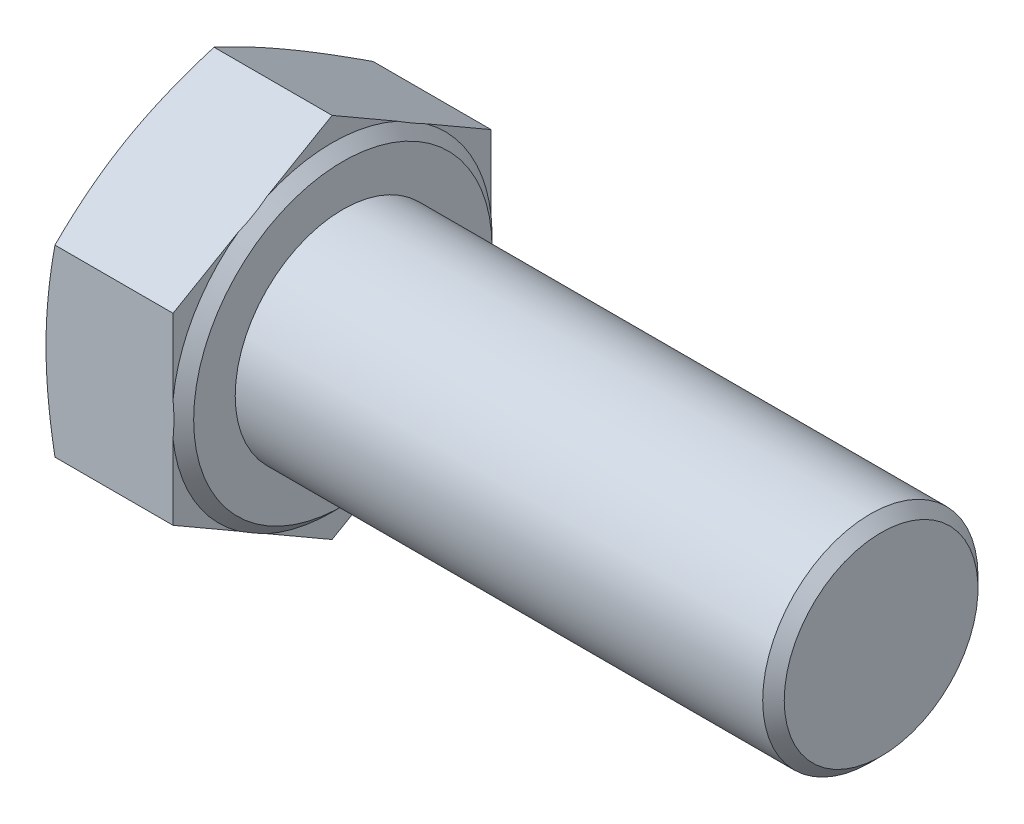
SolidWorks part; units mm, degrees
ref_plane "Front" through (0, 0, 0) normal (0, 0, 1) x (1, 0, 0)
ref_plane "Top" through (0, 0, 0) normal (0, 1, 0) x (1, 0, 0)
ref_plane "Right" through (0, 0, 0) normal (1, 0, 0) x (0, 0, -1)
other "Configuration Table"
sketch "Sketch2" plane through (0, 0, 0) normal (1, 0, 0) x (0, 0, -1)
  line L1 (8.865, -5.1182) -> (8.865, 5.1182)
  line L2 (8.865, 5.1182) -> (0, 10.2364)
  line L3 (0, 10.2364) -> (-8.865, 5.1182)
  line L4 (-8.865, 5.1182) -> (-8.865, -5.1182)
  line L5 (-8.865, -5.1182) -> (0, -10.2364)
  line L6 (0, -10.2364) -> (8.865, -5.1182)
  circle A0 centre (0, 0) radius 8.865 construction
extrude "BaseHead" add sketch "Sketch2" along normal blind 7.68
sketch "Sketch3" plane through (0, 0, 0) normal (0, 0, 1) x (1, 0, 0)
  line L0 (7.68, 10.2364) -> (7.68, 8.315)
  line L2 (7.68, 8.315) -> (7.08, 8.915)
  line L3 (7.08, 8.915) -> (7.08, 10.2364)
  line L5 (7.08, 10.2364) -> (7.68, 10.2364)
  line L6 (-0.9571, 0) -> (7.6478, 0) construction
  line L7 (7.68, 10.2364) -> (0, 10.2364) construction
  dimension "D1" = 45
  dimension "c" = 0.6
  dimension "Dw" = 16.63
revolve "BearingFace" cut sketch "Sketch3" angle 360 about L6
sketch "Sketch4" plane through (0, 0, 0) normal (0, 0, 1) x (1, 0, 0)
  line L0 (-0.4935, 0) -> (3.5626, 0) construction
  line L2 (0, 10.2364) -> (0.4992, 10.2364)
  line L4 (0.4992, 10.2364) -> (0, 8.865)
  line L6 (0, 8.865) -> (0, 10.2364)
  line L7 (7.08, 10.2364) -> (0, 10.2364) construction
revolve "HeadChamfer" cut sketch "Sketch4" angle 360 about L0
sketch "Sketch5" plane through (7.68, 0, 0) normal (1, 0, 0) x (0, 0, -1)
  circle A0 centre (0, 0) radius 6
extrude "BaseBody" add sketch "Sketch5" along normal blind 30
cosmetic thread "ThreadCosmetic1" parameters "D2"=10.106
chamfer "Chamfer1" distance 0.6 angle 45 1 edges at (37.68, 0, -6)
fillet "HeadFillet" [suppressed] radius 0.6
sketch "Sketch6" plane through (0, 0, 0) normal (0, 0, 1) x (1, 0, 0)
  line L0 (7.68, 6.947) -> (8.627, 6.947)
  line L1 (8.627, 6.947) -> (8.627, 6)
  line L2 (8.627, 6) -> (8.1535, 5.1799)
  line L3 (8.1535, 5.1799) -> (7.68, 6)
  line L4 (7.68, 6) -> (7.68, 6.947)
  line L5 (37.08, 6) -> (7.68, 6) construction
  line L6 (7.68, -8.315) -> (7.68, 8.315) construction
revolve "Cut-Revolve10" [suppressed] cut sketch "Sketch6" angle 360 about axis through (-0.9571, 0, 0) along (1, 0, 0)
pattern_linear "LPattern10" [suppressed] count 26
equation "\"D2@Sketch4\" = \"s@Sketch2\""
equation "\"D1@Chamfer1\" = 0.05 * \"d@Sketch5\""
equation "\"D1@Sketch6\" =  ( \"d@Sketch5\" - \"D2@ThreadCosmetic1\" )  / 2"
equation "\"pitch@LPattern10\" = \"D1@Sketch6\" * 1.2"
equation "\"D1@LPattern10\" = \"l@BaseBody\" / \"pitch@LPattern10\""
